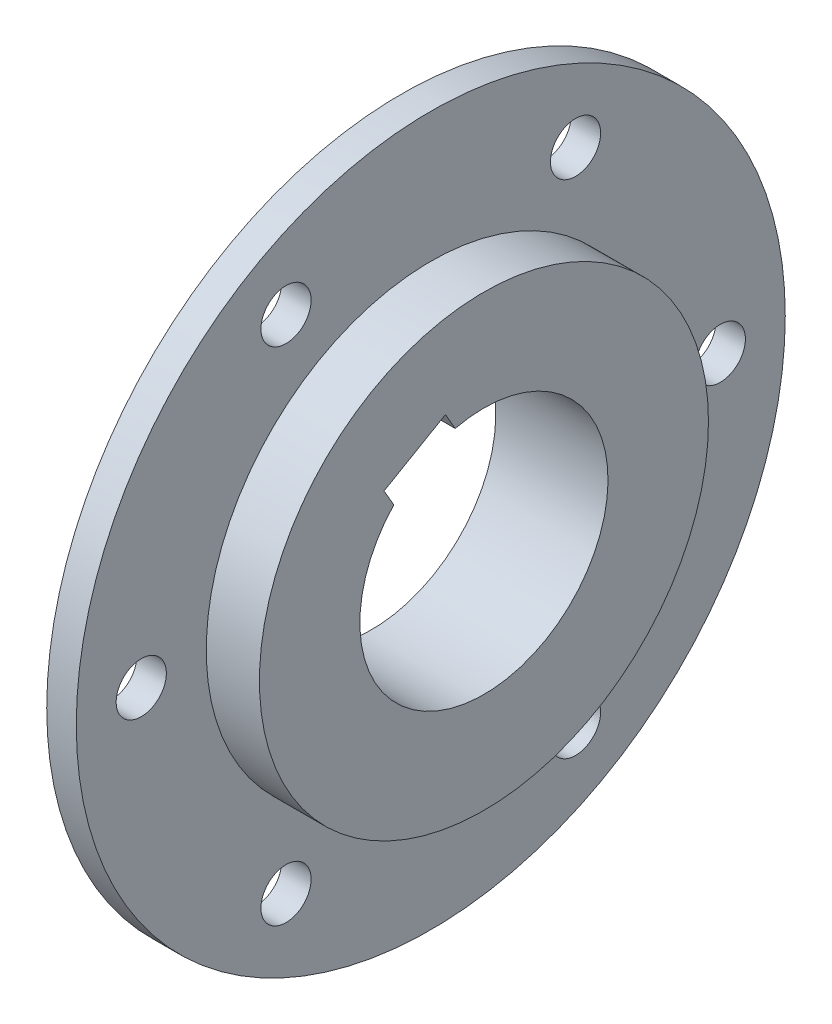
from build123d import *

# Parameters (mm, degrees)
EXTRUDE_1_DEPTH         = 14
EXTRUDE_1_DEPTH_BACK    = 5
SKETCH_1_R              = 38
SKETCH_2_R              = 60
SKETCH_2_R_2            = 38
EXTRUDE_2_DEPTH         = 5
CHAMFER_1_SIZE          = 1
HOLE_WIZARD_M10_1_D     = 8.5
HOLE_WIZARD_M10_1_DEPTH = 24.5
HOLE_WIZARD_M10_1_TIP   = 2.553657631


with BuildPart() as part:
    # 草图1 → 凸台-拉伸1 (new, two sides: drawn at the far end of the back side and taken through both)
    with BuildSketch(Plane(origin=(0, 0, 0), x_dir=(0, 0, -1), z_dir=(1, 0, 0)).offset(-EXTRUDE_1_DEPTH_BACK)):
        Circle(SKETCH_1_R)
        with BuildLine():
            Line((-4.866153476, 20.428425058), (-6.516153476, 23.28630889))
            Line((-6.516153476, 23.28630889), (-16.908458321, 17.28630889))
            Line((-16.908458321, 17.28630889), (-15.258458321, 14.428425058))
            ThreePointArc((-15.258458321, 14.428425058), (10.5, -18.186533479), (-4.866153476, 20.428425058))
        make_face(mode=Mode.SUBTRACT)
    extrude(amount=EXTRUDE_1_DEPTH + EXTRUDE_1_DEPTH_BACK)

    # 草图2 → 凸台-拉伸2 (add)
    with BuildSketch(Plane(origin=(0, 0, 0), x_dir=(0, 0, -1), z_dir=(1, 0, 0))):
        Circle(SKETCH_2_R)
        Circle(SKETCH_2_R_2, mode=Mode.SUBTRACT)
    extrude(amount=EXTRUDE_2_DEPTH)

    # 倒角1
    chamfer_1_edges = [part.edges().sort_by_distance(p)[0] for p in [
        (-5, 0, 38),
    ]]
    chamfer(chamfer_1_edges, length=CHAMFER_1_SIZE)

    # M10 螺纹孔1
    with Locations(Plane.ZY):
        with Locations((24.5, 42.435244785), (49, 0), (24.5, -42.435244785), (-24.5, -42.435244785), (-49, 0), (-24.5, 42.435244785)):
            Hole(HOLE_WIZARD_M10_1_D / 2, depth=HOLE_WIZARD_M10_1_DEPTH)
            with Locations((0, 0, -(HOLE_WIZARD_M10_1_DEPTH + HOLE_WIZARD_M10_1_TIP / 2))):  # 118° drill point
                Cone(0, HOLE_WIZARD_M10_1_D / 2, HOLE_WIZARD_M10_1_TIP, mode=Mode.SUBTRACT)


solid = part.part
